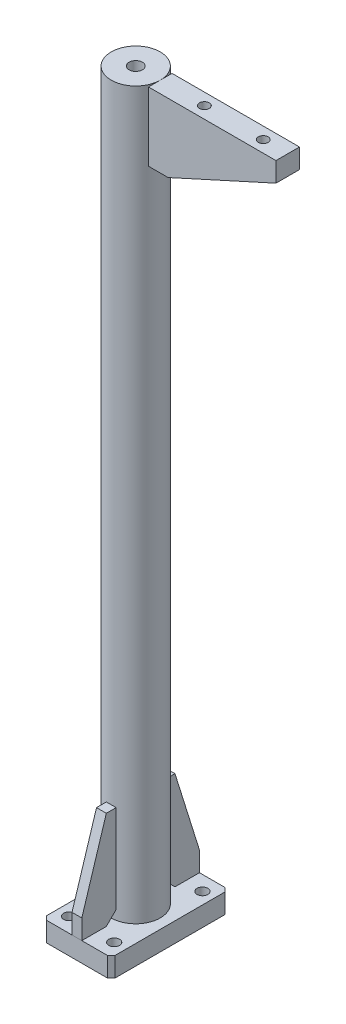
SolidWorks part; units mm, degrees
material "45#"
ref_plane "前基準面" through (0, 0, 0) normal (0, 0, 1) x (1, 0, 0)
ref_plane "上基準面" through (0, 0, 0) normal (0, 1, 0) x (1, 0, 0)
ref_plane "右基準面" through (0, 0, 0) normal (1, 0, 0) x (0, 0, -1)
sketch "草图1" plane through (0, 0, 0) normal (0, 1, 0) x (1, 0, 0)
  circle A0 centre (0, 0) radius 12.5
  dimension "D1" = 25
extrude "凸台-拉伸1" add sketch "草图1" along normal blind 370
sketch "草图2" plane through (0, 0, 0) normal (0, -1, 0) x (1, 0, 0)
  line L1 (17.5, -30) -> (-17.5, -30)
  line L2 (17.5, -30) -> (17.5, 30)
  line L3 (17.5, 30) -> (-17.5, 30)
  line L4 (-17.5, -30) -> (-17.5, 30)
  line L5 (17.5, -30) -> (-17.5, 30) construction
  line L6 (17.5, 30) -> (-17.5, -30) construction
  point P0 (0, 0)
  dimension "D1" = 60
  dimension "D2" = 35
extrude "凸台-拉伸2" add sketch "草图2" along normal blind 10 separate body
sketch "草图3" plane through (0, 0, 0) normal (0, 0, 1) x (1, 0, 0)
  line L0 (0, 0) -> (0, 426.7494) construction
  line L1 (12.5, 370) -> (77.5, 370)
  line L2 (77.5, 370) -> (77.5, 360)
  line L3 (77.5, 360) -> (22.5, 335)
  line L4 (22.5, 335) -> (12.5, 335)
  line L5 (12.5, 0) -> (12.5, 370) construction
  line L6 (12.5, 335) -> (12.5, 370)
  dimension "D1" = 10
  dimension "D2" = 10
  dimension "D3" = 65
  dimension "D4" = 35
extrude "凸台-拉伸3" add sketch "草图3" along normal mid plane 12 separate body
hole_wizard "M8 螺纹孔1" positions "草图4" profile "草图5" tap size "M8" standard "GB"
sketch "草图4" plane through (0, 370, 0) normal (0, 1, 0) x (1, 0, 0)
  point P0 (0, 0)
sketch "草图5" plane through (0, 370, 0) normal (1, 0, 0) x (0, 0, 1)
  line L0 (0, 0) -> (0, 21.7929)
  line L1 (0, 21.7929) -> (3.4, 19.75)
  line L2 (3.4, 19.75) -> (3.4, 0)
  line L5 (3.4, 0) -> (0, 0)
  line L10 (0, 21.7929) -> (-3.4, 19.75) construction
  line L11 (0, -6.35) -> (0, 107.95) construction
  dimension "螺纹孔钻头直径" = 6.8
  dimension "螺纹孔钻头深度" = 19.75
  dimension "导头角度" = 118
cosmetic thread "孔螺蚊线1" parameters "D1"=16, "D2"=8
hole_wizard "M6 螺纹孔1" positions "草图6" profile "草图7" tap size "M6" standard "GB"
sketch "草图6" plane through (0, 370, 0) normal (0, 1, 0) x (1, 0, 0)
  line L0 (0, 0) -> (85.34, 0) construction
  line L2 (0, 0) -> (0, 41.2455) construction
  point P0 (35, 0)
  point P2 (65, 0)
  dimension "D1" = 35
  dimension "D2" = 30
sketch "草图7" plane through (35, 370, 0) normal (1, 0, 0) x (0, 0, 1)
  line L0 (0, 0) -> (0, 16.5022)
  line L1 (0, 16.5022) -> (2.5, 15)
  line L2 (2.5, 15) -> (2.5, 0)
  line L5 (2.5, 0) -> (0, 0)
  line L10 (0, 16.5022) -> (-2.5, 15) construction
  line L11 (0, -6.35) -> (0, 107.95) construction
  dimension "螺纹孔钻头直径" = 5
  dimension "螺纹孔钻头深度" = 15
  dimension "导头角度" = 118
cosmetic thread "孔螺蚊线2" parameters "D1"=12, "D2"=6
cosmetic thread "孔螺蚊线3" parameters "D1"=12, "D2"=6
sketch "草图8" plane through (0, 0, 0) normal (1, 0, 0) x (0, 0, -1)
  line L0 (30, 0) -> (30, 10)
  line L1 (30, 10) -> (17.5, 50)
  line L2 (17.5, 50) -> (12.5, 50)
  line L3 (12.5, 0) -> (12.5, 370) construction
  line L4 (12.5, 50) -> (12.5, 5)
  line L5 (-12.5, 0) -> (12.5, 0) construction
  line L6 (17.5, 0) -> (30, 0)
  line L7 (12.5, 5) -> (17.5, 0)
  line L8 (0, 0) -> (0, 93.607) construction
  line L9 (-12.5, 5) -> (-17.5, 0)
  line L10 (-17.5, 0) -> (-30, 0)
  line L11 (-12.5, 50) -> (-12.5, 5)
  line L12 (-17.5, 50) -> (-12.5, 50)
  line L13 (-30, 10) -> (-17.5, 50)
  line L14 (-30, 0) -> (-30, 10)
  point P8 (12.5, 0)
  point P15 (-12.5, 0)
  dimension "D1" = 10
  dimension "D2" = 5
  dimension "D4" = 50
extrude "凸台-拉伸4" add sketch "草图8" along normal mid plane 5 separate body
hole_wizard "M5 间隙孔1" positions "草图9" profile "草图10" hole size "M5" standard "GB"
sketch "草图9" plane through (0, -10, 0) normal (0, -1, 0) x (-1, 0, 0)
  line L0 (0, 0) -> (0, 38.1831) construction
  line L2 (0, 0) -> (24.1889, 0) construction
  line L4 (17.5, -30) -> (17.5, 30) construction
  line L5 (17.5, 30) -> (-17.5, 30) construction
  point P0 (-11.5, 22.5)
  point P2 (11.5, 22.5)
  point P14 (11.5, -22.5)
  point P15 (-11.5, -22.5)
  dimension "D1" = 6
  dimension "D2" = 7.5
sketch "草图10" plane through (11.5, -10, -22.5) normal (1, 0, 0) x (0, 0, -1)
  line L0 (0, 0) -> (0, 16.6524)
  line L1 (0, 16.6524) -> (2.75, 15)
  line L2 (2.75, 15) -> (2.75, 0)
  line L5 (2.75, 0) -> (0, 0)
  line L10 (0, 16.6524) -> (-2.75, 15) construction
  line L11 (0, -6.35) -> (0, 107.95) construction
  dimension "孔直径" = 5.5
  dimension "孔深度" = 15
  dimension "导头角度" = 118
chamfer "倒角1" distance 2 angle 45 4 edges at (-17.5, -5, -30) (-17.5, -5, 30) (17.5, -5, -30) (17.5, -5, 30)
